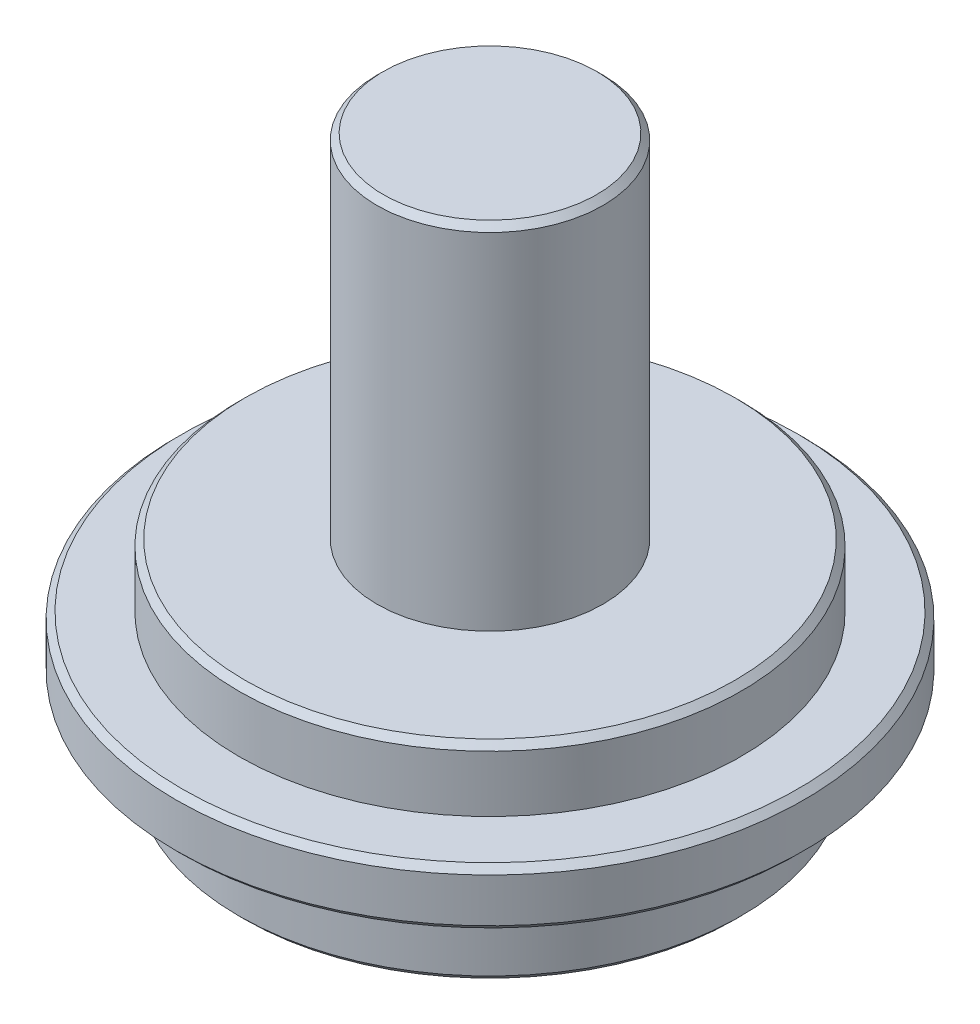
SolidWorks part; units mm, degrees
material "45"
ref_plane "Front Plane" through (0, 0, 0) normal (0, 0, 1) x (1, 0, 0)
ref_plane "Top Plane" through (0, 0, 0) normal (0, 1, 0) x (1, 0, 0)
ref_plane "Right Plane" through (0, 0, 0) normal (1, 0, 0) x (0, 0, -1)
sketch "Sketch1" plane through (0, 0, 0) normal (0, 0, 1) x (1, 0, 0)
  line L0 (258.3143, -567) -> (258.3143, -595)
  line L1 (258.3143, -595) -> (269.3143, -595)
  line L2 (269.3143, -595) -> (269.3143, -600)
  line L3 (269.3143, -600) -> (274.3143, -600)
  line L4 (289.5143, -600) -> (-290.8857, -600) construction
  line L5 (274.3143, -600) -> (274.3143, -604.5)
  line L6 (274.3143, -604.5) -> (269.3143, -604.5)
  line L7 (269.3143, -604.5) -> (269.3143, -611.5)
  line L8 (269.3143, -611.5) -> (249.3143, -611.5)
  line L9 (249.3143, -567) -> (249.3143, -611.5) construction
  line L10 (258.3143, -567) -> (249.3143, -567)
  line L12 (249.3143, -567) -> (249.3143, -611.5)
  dimension "D1" = 20
  dimension "D2" = 5
  dimension "D3" = 4.5
  dimension "D4" = 7
  dimension "D5" = 5
  dimension "D6" = 9
  dimension "D7" = 28
revolve "Revolve1" add sketch "Sketch1" angle 360 about L9
chamfer "Chamfer1" distance 0.5 angle 45 5 edges at (249.3143, -611.5, 20) (249.3143, -604.5, 25) (249.3143, -600, 25) (249.3143, -595, 20) (249.3143, -567, 9)
